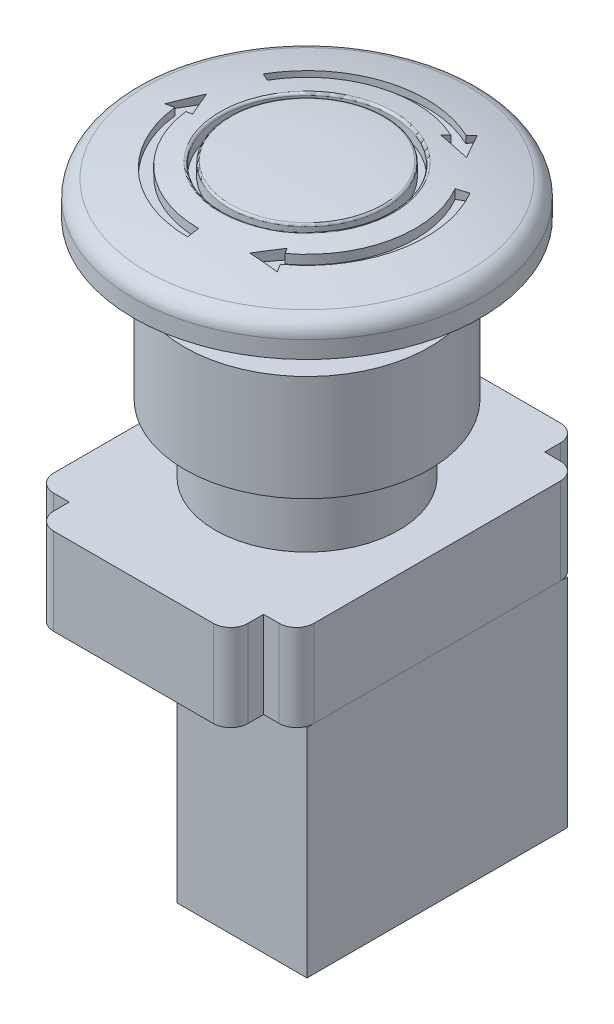
from build123d import *

# Parameters (mm, degrees)
SKETCH_2_W          = 30
SKETCH_2_H          = 40
EXTRUDE_1_DEPTH     = 10
SKETCH_3_W          = 15
SKETCH_3_H          = 30
EXTRUDE_2_DEPTH     = 25
SKETCH_7_W          = 3.8
SKETCH_7_H          = 3.8
CUT_EXTRUDE_2_DEPTH = 10
FILLET_1_R          = 2
FILLET_2_R          = 2
SKETCH_8_R          = 9.75
SKETCH_8_R_2        = 9
CUT_EXTRUDE_4_DEPTH = 5
CUT_EXTRUDE_5_DEPTH = 5
FILLET_3_R          = 0.25


with BuildPart() as part:
    # 草图1 → 旋转1 (revolve)
    with BuildSketch(Plane.XY, mode=Mode.PRIVATE) as revolve_1_sk:
        with BuildLine():
            Line((14.1, 20), (11, 20))
            Line((11, 20), (11, 29))
            ThreePointArc((11, 29), (14.791548694, 28.29957327), (18.538082764, 27.388572956))
            Line((18.538082764, 27.388572956), (18.538082764, 25.871274116))
            Line((18.538082764, 25.871274116), (20, 25.871274116))
            Line((20, 25.871274116), (20, 29.371274116))
            ThreePointArc((20, 29.371274116), (10.09698248, 31.423503879), (0, 32))
            Line((0, 32), (0, 0))
            Line((0, 0), (10.6, 0))
            Line((10.6, 0), (10.6, 7.8))
            Line((10.6, 7.8), (14.1, 7.8))
            Line((14.1, 7.8), (14.1, 20))
        make_face()
    revolve(revolve_1_sk.sketch.rotate(Axis((0, 0, 0), (0, 1, 0)), 90), axis=Axis((0, 0, 0), (0, 1, 0)))

    # 圆角2
    fillet_2_edges = [part.edges().sort_by_distance(p)[0] for p in [
        (0, 29.371274116, 20),
    ]]
    fillet(fillet_2_edges, radius=FILLET_2_R)

    # 草图8 → 切除-拉伸4 (cut)
    with BuildSketch(Plane(origin=(0, 30, 0), x_dir=(-1, 0, 0), z_dir=(0, 1, 0))):
        with Locations(Location((0, 0, 0), (0, 0, 270))):
            Circle(SKETCH_8_R)
        with Locations(Location((0, 0, 0), (0, 0, 270))):
            Circle(SKETCH_8_R_2, mode=Mode.SUBTRACT)
    extrude(amount=CUT_EXTRUDE_4_DEPTH, mode=Mode.SUBTRACT)

    # 草图9 → 切除-拉伸5 (cut)
    with BuildSketch(Plane(origin=(0, 30, 0), x_dir=(-1, 0, 0), z_dir=(0, 1, 0))):
        with BuildLine():
            Line((11.907849302, -6.875), (10.825317547, -6.25))
            ThreePointArc((10.825317547, -6.25), (3.79320889, -11.910565323), (-5.217256711, -11.359147521))
            Line((-5.217256711, -11.359147521), (-4.772623337, -10.647734123))
            Line((-4.772623337, -10.647734123), (-8.270350551, -10.108436975))
            Line((-8.270350551, -10.108436975), (-6.39051478, -13.236360431))
            Line((-6.39051478, -13.236360431), (-5.884720677, -12.427089867))
            ThreePointArc((-5.884720677, -12.427089867), (4.095844856, -13.125797306), (11.907849302, -6.875))
        make_face()
        with BuildLine():
            Line((0, 12.5), (0, 13.75))
            ThreePointArc((0, 13.75), (9.153426635, 10.260471765), (13.660869169, 1.563059031))
            Line((13.660869169, 1.563059031), (14.836795077, 1.563059031))
            Line((14.836795077, 1.563059031), (13.055774782, -1.473434586))
            Line((13.055774782, -1.473434586), (11.625119135, 1.563059031))
            Line((11.625119135, 1.563059031), (12.401888827, 1.563059031))
            ThreePointArc((12.401888827, 1.563059031), (8.26776155, 9.375186342), (0, 12.5))
        make_face()
        with BuildLine():
            Line((-10.825317547, -6.25), (-11.907849302, -6.875))
            ThreePointArc((-11.907849302, -6.875), (-13.448042492, 2.865772692), (-8.070484546, 11.132375272))
            Line((-8.070484546, 11.132375272), (-8.478555156, 11.907849302))
            Line((-8.478555156, 11.907849302), (-5.333788149, 11.907849302))
            Line((-5.333788149, 11.907849302), (-7.194072858, 9.466892667))
            Line((-7.194072858, 9.466892667), (-7.481781605, 10.013637901))
            ThreePointArc((-7.481781605, 10.013637901), (-12.243935204, 2.517151309), (-10.825317547, -6.25))
        make_face()
    extrude(amount=CUT_EXTRUDE_5_DEPTH, mode=Mode.SUBTRACT)

    # 圆角3
    fillet_3_edges = [part.edges().sort_by_distance(p)[0] for p in [
        (1e-09, 31.468211744, 9.749999987),
        (2e-09, 31.558721819, 9),
    ]]
    fillet(fillet_3_edges, radius=FILLET_3_R)


with BuildPart() as body_2:
    # 草图2 → 拉伸1 (new body)
    with BuildSketch(Plane.XZ):
        Rectangle(SKETCH_2_W, SKETCH_2_H)
    extrude(amount=EXTRUDE_1_DEPTH)

    # 草图7 → 切除-拉伸2 (cut)
    with BuildSketch(Plane(origin=(0, 0, 0), x_dir=(-1, 0, 0), z_dir=(0, 1, 0))):
        with Locations((-13.1, 18.1)):
            Rectangle(SKETCH_7_W, SKETCH_7_H)
        with Locations((13.1, 18.1)):
            Rectangle(SKETCH_7_W, SKETCH_7_H)
        with Locations((13.1, -18.1)):
            Rectangle(SKETCH_7_W, SKETCH_7_H)
        with Locations((-13.1, -18.1)):
            Rectangle(SKETCH_7_W, SKETCH_7_H)
    extrude(amount=-CUT_EXTRUDE_2_DEPTH, mode=Mode.SUBTRACT)

    # 圆角1
    fillet_1_edges = [body_2.edges().sort_by_distance(p)[0] for p in [
        (15, -5, 16.2),
        (11.2, -5, 20),
        (-11.2, -5, 20),
        (-15, -5, 16.2),
        (-15, -5, -16.2),
        (-11.2, -5, -20),
        (11.2, -5, -20),
        (15, -5, -16.2),
    ]]
    fillet(fillet_1_edges, radius=FILLET_1_R)


with BuildPart() as body_3:
    # 草图3 → 拉伸2 (new body)
    with BuildSketch(Plane.XZ.offset(10)):
        with Locations((7.5, 0)):
            Rectangle(SKETCH_3_W, SKETCH_3_H)
    extrude(amount=EXTRUDE_2_DEPTH)


solid = Compound([part.part, body_2.part, body_3.part])
